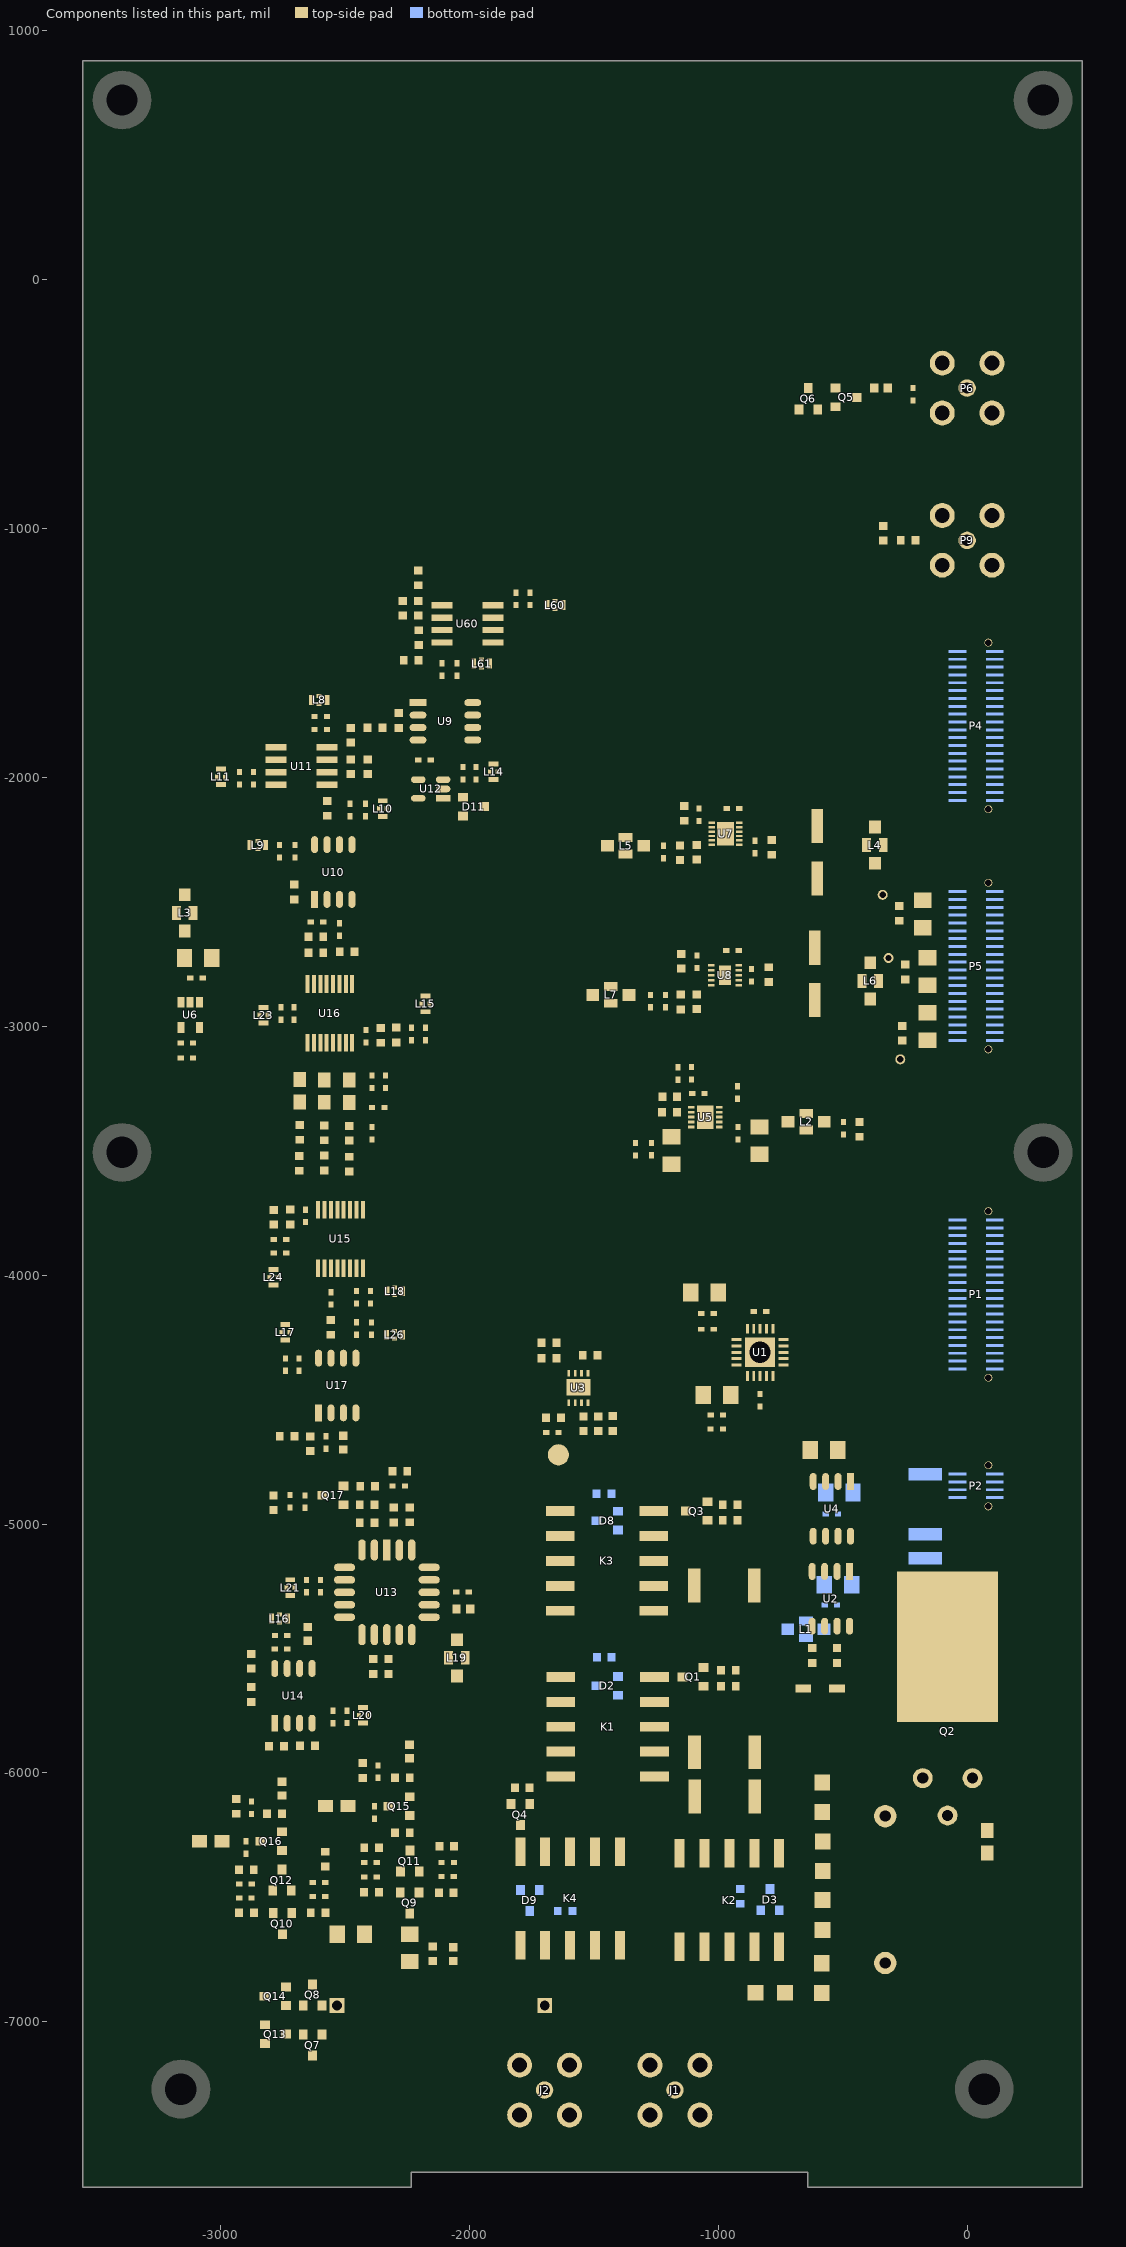
[diagram p0: the components of this part, seen from the top]
# Altium PCB MISC109358.PcbDoc (part 7 of 7)
Units mil, origin at the board's own origin, x right, y up, seen from the top; angles counter-clockwise.
Board outline 4015.75 x 8543.31 mil, 4 copper layers (TopLayer, GND, POWER, BottomLayer), stack 33.234 mil thick; 299 components, 170 nets, 998 pads, 2318 vias.

## Polygon pours and split planes (outlines as drawn) (continued)
+5V on POWER (split plane): -861.09,-1578.18 -861.09,-2676.82 -1464.65,-3280.39 -1466.25,-3282.48 -1467.26,-3284.91 -1467.61,-3287.52 -1467.61,-5990.34 -2168.7,-6691.43 -3532.9,-6691.43 -3532.9,-6144.61 -3024.7,-6144.61 -2941.61,-6227.7 -2941.61,-6369.52 -2941.26,-6372.13 -2940.25,-6374.56 -2938.65,-6376.65 -2894.65,-6420.65 -2892.56,-6422.25 -2890.13,-6423.26 -2887.52,-6423.61 -2789.52,-6423.61 -2786.91,-6423.26 -2784.48,-6422.25 -2782.39,-6420.65 -2741.39,-6379.65 -2739.78,-6377.56 -2738.78,-6375.13 -2738.43,-6372.52 -2738.43,-6061.7 -2691.34,-6014.61 -2539.7,-6014.61 -2476.61,-6077.7 -2476.61,-6254.52 -2476.26,-6257.13 -2475.25,-6259.56 -2473.65,-6261.65 -2424.65,-6310.65 -2422.56,-6312.25 -2420.13,-6313.26 -2417.52,-6313.61 -2327.52,-6313.61 -2324.91,-6313.26 -2322.48,-6312.25 -2320.39,-6310.65 -2282.39,-6272.65 -2280.78,-6270.56 -2279.78,-6268.13 -2279.43,-6265.52 -2279.43,-5742.52 -2279.78,-5739.91 -2280.78,-5737.48 -2282.39,-5735.39 -2409.91,-5607.87 -2412,-5606.26 -2414.43,-5605.26 -2417.04,-5604.91 -2867.82,-5604.91 -2923.91,-5548.82 -2923.91,-5397.18 -2887.34,-5360.61 -2660.52,-5360.61 -2657.91,-5360.26 -2655.48,-5359.25 -2653.39,-5357.65 -2628.39,-5332.65 -2626.78,-5330.56 -2625.78,-5328.13 -2625.43,-5325.52 -2625.43,-4502.7 -2521.34,-4398.61 -2237.52,-4398.61 -2234.91,-4398.26 -2232.48,-4397.25 -2230.39,-4395.65 -2163.39,-4328.65 -2161.78,-4326.56 -2160.78,-4324.13 -2160.43,-4321.52 -2160.43,-4051.52 -2160.78,-4048.91 -2161.78,-4046.48 -2163.39,-4044.39 -2208.39,-3999.39 -2210.48,-3997.78 -2212.91,-3996.78 -2215.52,-3996.43 -2455.52,-3996.43 -2458.13,-3996.78 -2459.14,-3997.19 -2460.56,-3997.78 -2462.65,-3999.39 -2643.18,-4179.91 -2770.82,-4179.91 -2884.91,-4065.82 -2884.91,-3226.18 -2775.39,-3116.65 -2773.78,-3114.56 -2772.78,-3112.13 -2772.43,-3109.52 -2772.43,-2881.52 -2772.78,-2878.91 -2773.78,-2876.48 -2775.39,-2874.39 -3183.43,-2466.34 -3183.43,-2365.7 -3059.82,-2242.09 -2522.18,-2242.09 -2370.13,-2394.13 -2368.04,-2395.74 -2365.61,-2396.74 -2363,-2397.09 -1474,-2397.09 -1471.39,-2396.74 -1468.96,-2395.74 -1466.87,-2394.13 -1410.87,-2338.13 -1409.26,-2336.04 -1408.97,-2335.33 -1408.26,-2333.61 -1407.91,-2331 -1407.91,-1821.04 -1408.26,-1818.43 -1408.55,-1817.72 -1409.26,-1816 -1410.87,-1813.91 -1446.39,-1778.39 -1712.91,-1511.87 -1715,-1510.26 -1717.43,-1509.26 -1720.04,-1508.91 -1958,-1508.91 -1960.61,-1509.26 -1963.04,-1510.26 -1965.13,-1511.87 -2179.7,-1726.43 -3532.9,-1726.43 -3532.9,-1198.61 -1240.66,-1198.61
-5V on POWER (split plane): -1460.65,-1792.65 -1428.09,-1825.22 -1428.09,-2326.82 -1478.18,-2376.91 -2358.82,-2376.91 -2510.87,-2224.87 -2512.96,-2223.26 -2515.39,-2222.26 -2518,-2221.91 -3064,-2221.91 -3066.61,-2222.26 -3069.04,-2223.26 -3071.13,-2224.87 -3200.65,-2354.39 -3202.25,-2356.48 -3203.26,-2358.91 -3203.61,-2361.52 -3203.61,-2470.52 -3203.26,-2473.13 -3202.25,-2475.56 -3200.65,-2477.65 -2792.61,-2885.7 -2792.61,-3105.34 -2902.13,-3214.87 -2903.73,-3216.96 -2904.74,-3219.39 -2905.09,-3222 -2905.09,-4070 -2904.74,-4072.61 -2903.73,-4075.04 -2902.13,-4077.13 -2782.13,-4197.13 -2780.04,-4198.74 -2777.61,-4199.74 -2775,-4200.09 -2639,-4200.09 -2636.39,-4199.74 -2633.96,-4198.74 -2631.87,-4197.13 -2451.34,-4016.61 -2219.7,-4016.61 -2180.61,-4055.7 -2180.61,-4317.34 -2241.7,-4378.43 -2525.52,-4378.43 -2528.13,-4378.78 -2530.56,-4379.78 -2532.65,-4381.39 -2642.65,-4491.39 -2644.25,-4493.48 -2645.26,-4495.91 -2645.61,-4498.52 -2645.61,-5321.34 -2664.7,-5340.43 -2891.52,-5340.43 -2894.13,-5340.78 -2896.56,-5341.78 -2898.65,-5343.39 -2941.13,-5385.87 -2942.73,-5387.96 -2943.74,-5390.39 -2944.09,-5393 -2944.09,-5553 -2943.74,-5555.61 -2942.73,-5558.04 -2941.13,-5560.13 -2879.13,-5622.13 -2877.04,-5623.74 -2874.61,-5624.74 -2872,-5625.09 -2421.22,-5625.09 -2299.61,-5746.7 -2299.61,-6261.34 -2331.7,-6293.43 -2413.34,-6293.43 -2456.43,-6250.34 -2456.43,-6073.52 -2456.78,-6070.91 -2457.78,-6068.48 -2459.39,-6066.39 -2528.39,-5997.39 -2530.48,-5995.78 -2532.91,-5994.78 -2535.52,-5994.43 -2695.52,-5994.43 -2698.13,-5994.78 -2700.56,-5995.78 -2702.65,-5997.39 -2755.65,-6050.39 -2757.25,-6052.48 -2758.26,-6054.91 -2758.61,-6057.52 -2758.61,-6368.34 -2793.7,-6403.43 -2883.34,-6403.43 -2921.43,-6365.34 -2921.43,-6223.52 -2921.78,-6220.91 -2922.78,-6218.48 -2924.39,-6216.39 -3013.39,-6127.39 -3015.48,-6125.78 -3017.91,-6124.78 -3020.52,-6124.43 -3532.9,-6124.43 -3532.9,-1746.61 -2175.52,-1746.61 -2172.91,-1746.26 -2170.48,-1745.25 -2168.39,-1743.65 -1953.82,-1529.09 -1724.22,-1529.09

## Keep-outs
KeepOutLayer:
  lines w10: -3553,-7664 -2233.7,-7664 -2233.7,-7604.94 -640.3,-7604.94 -640.3,-7664 462.75,-7664 462.75,879.31 -3553,879.31 -3553,-7664 ; -397.52,-5931.52 -1.52,-5931.52 -1.52,-5819.52 -301.14,-5819.52 -301.14,-4672.52 121.48,-4672.52 121.48,-4572.52 -397.52,-4572.52 -397.52,-4878.52 -397.52,-5931.52

## Other copper
TopLayer:
  pour cut-out: -2175.52,-1512.52 -2175.35,-1512.69 -2175.35,-1578.69 -2170.52,-1583.52 -2141.52,-1583.52 -2136.52,-1578.52 -2136.52,-1508.52 -2145.52,-1499.52 -2169.37,-1499.52 -2175.52,-1505.67
  pour cut-out: -2518.52,-2112.52 -2584.69,-2112.69 -2589.52,-2117.52 -2589.52,-2146.52 -2584.52,-2151.52 -2514.52,-2151.52 -2514.52,-2112.52
  pour cut-out: -2507.52,-1824.52 -2507.69,-1824.35 -2507.69,-1758.35 -2512.52,-1753.52 -2541.52,-1753.52 -2546.52,-1758.52 -2546.52,-1828.52 -2537.52,-1837.52 -2513.67,-1837.52 -2507.52,-1831.37
  pour cut-out: -822.52,-6401.52 -822.52,-6611.52 -786.52,-6647.52 -724.8,-6647.52 -705.14,-6627.86 -705.14,-6395.9 -717.52,-6383.52 -804.52,-6383.52
  pour cut-out: -2775,-7007.58 -2641.24,-7007.24 -2622.52,-6988.52 -2642.46,-6968.58 -2779,-6968.58 -2788,-6977.58 -2788,-7001.43 -2781.85,-7007.58
  pour cut-out: -2699.52,-6818.52 -2699.35,-6818.69 -2699.35,-6884.69 -2694.52,-6889.52 -2665.52,-6889.52 -2660.52,-6884.52 -2660.52,-6814.52 -2669.52,-6805.52 -2693.37,-6805.52 -2699.52,-6811.67
  pour cut-out: -1767.52,-6542.52 -1767.35,-6542.69 -1767.35,-6608.69 -1762.52,-6613.52 -1733.52,-6613.52 -1728.52,-6608.52 -1728.52,-6538.52 -1737.52,-6529.52 -1761.37,-6529.52 -1767.52,-6535.67
GND (plane layer: these items are gaps in the copper):
  region: -301.14,-4672.52 -301.14,-5819.52 -1.52,-5819.52 -1.52,-6093.52 -384.52,-6093.52 -384.52,-6263.52 226.48,-6263.52 226.48,-4972.52 33.48,-4972.52 33.48,-4672.52
POWER (plane layer: these items are gaps in the copper):
  region: -301.14,-4672.52 -301.14,-5819.52 -1.52,-5819.52 -1.52,-6093.52 -384.52,-6093.52 -384.52,-6263.52 226.48,-6263.52 226.48,-4972.52 33.48,-4972.52 33.48,-4672.52
  lines w20: -3549.52,-6701.52 -2164.52,-6701.52 -1457.52,-5994.52 -1457.52,-3287.52 -851,-2681 -851,-1574 -1236.48,-1188.52 -3544.52,-1188.52 ; -3548.52,-6134.52 -3020.52,-6134.52 -2931.52,-6223.52 -2931.52,-6369.52 -2887.52,-6413.52 -2789.52,-6413.52 -2748.52,-6372.52 -2748.52,-6057.52 -2695.52,-6004.52 -2535.52,-6004.52 -2466.52,-6073.52 -2466.52,-6254.52 -2417.52,-6303.52 -2327.52,-6303.52 -2289.52,-6265.52 -2289.52,-5742.52 -2417.04,-5615 -2872,-5615 -2934,-5553 -2934,-5393 -2891.52,-5350.52 -2758.52,-5350.52 -2660.52,-5350.52 -2635.52,-5325.52 -2635.52,-4498.52 -2525.52,-4388.52 -2237.52,-4388.52 -2170.52,-4321.52 -2170.52,-4051.52 -2215.52,-4006.52 -2455.52,-4006.52 -2639,-4190 -2775,-4190 -2895,-4070 -2895,-3222 -2782.52,-3109.52 -2782.52,-2881.52 -3193.52,-2470.52 -3193.52,-2361.52 -3064,-2232 -2518,-2232 -2363,-2387 -1474,-2387 -1418,-2331 -1418,-1821.04 -1453.52,-1785.52 -1720.04,-1519 -1958,-1519 -2175.52,-1736.52 -3538.52,-1736.52

## Silkscreen, mask and mechanical layers (free items; w line width, h text height)
TopSolder:
  lines w157.48: -3395.52,-7506.52 305.27,-7506.52 305.27,287.48 -3395.52,287.48 -3395.52,-3506.52 -3395.52,-7506.52
BottomSolder:
  lines w157.48: -3394.52,-7506.52 306.27,-7506.52 306.27,287.48 -3394.52,287.48 -3394.52,-3506.52 -3394.52,-7506.52